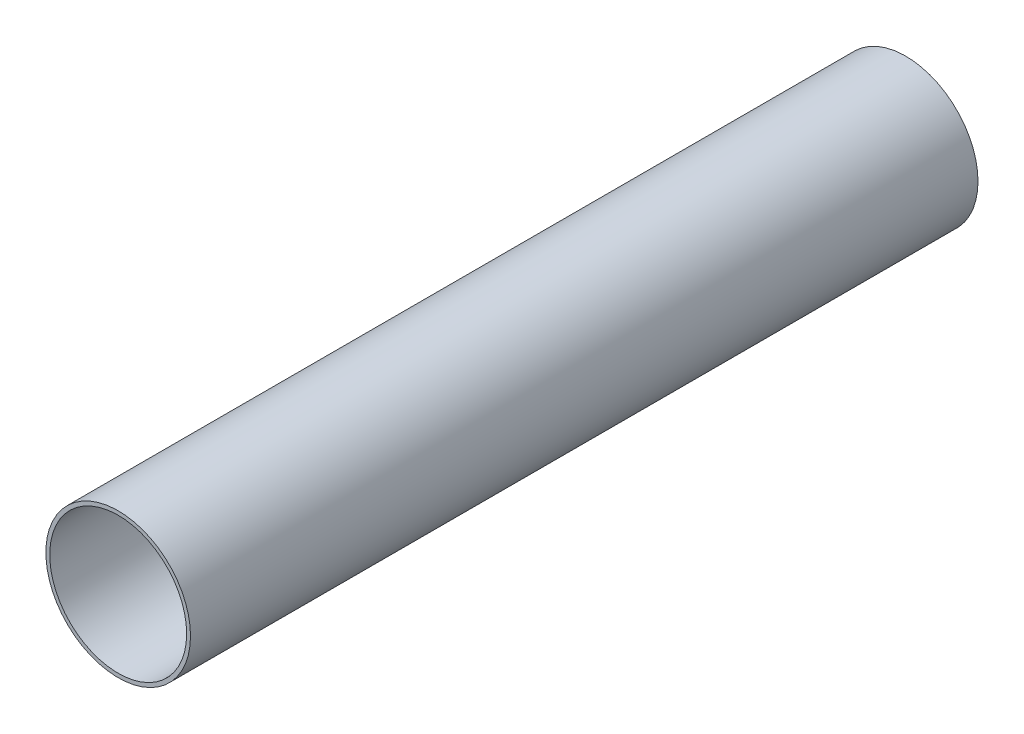
SolidWorks part; units mm, degrees
material "Q235"
ref_plane "Front Plane" through (0, 0, 0) normal (0, 0, 1) x (1, 0, 0)
ref_plane "Top Plane" through (0, 0, 0) normal (0, 1, 0) x (1, 0, 0)
ref_plane "Right Plane" through (0, 0, 0) normal (1, 0, 0) x (0, 0, -1)
sketch "Sketch1" plane through (0, 0, 0) normal (0, 0, 1) x (1, 0, 0)
  circle A0 centre (0, 0) radius 22.5
  circle A1 centre (0, 0) radius 21.3
  dimension "D1" = 45
  dimension "D2" = 1.2
extrude "Boss-Extrude1" add sketch "Sketch1" along normal blind 245
